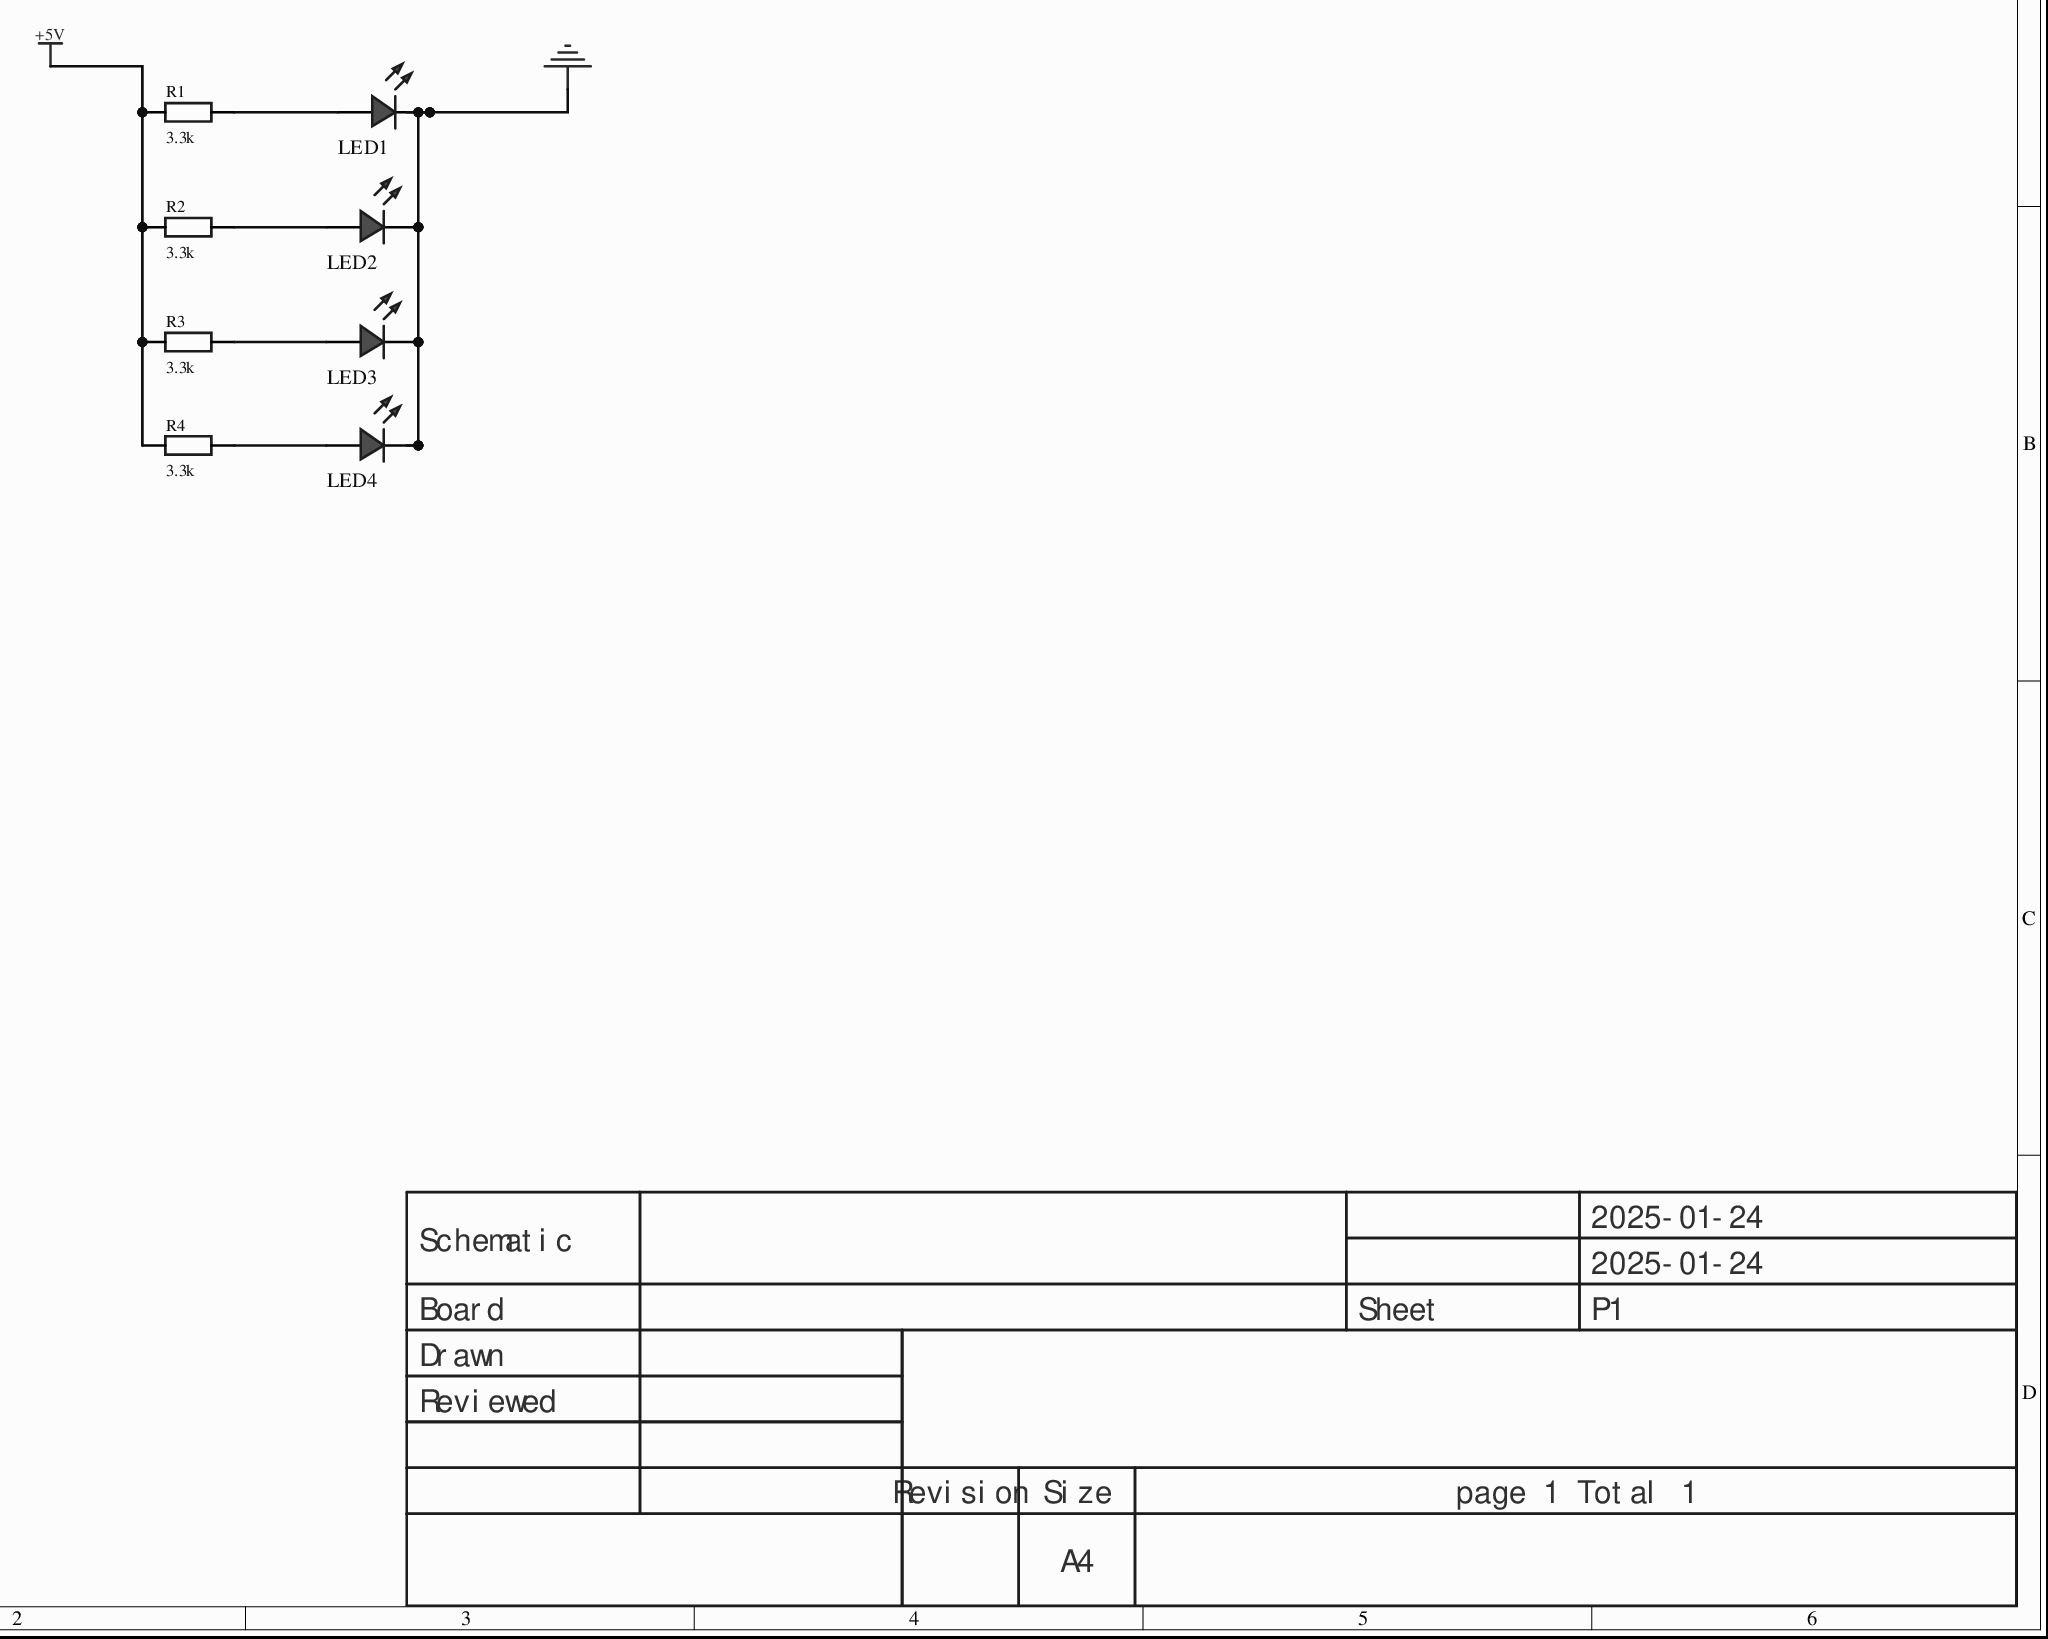
[diagram p0: MISC51832-3.schdoc]
# Altium project MISC51832-2.PrjPcb
1 sheet, 8 parts. Net scope: global (net labels, ports and power ports of the same name join across sheets).
Board file: MISC51832.pcbdoc

## Sheet MISC51832-3.schdoc
size 297 x 209 mm; Version: V1.0; @Project Name: MISC51832; @Page Count: 1; @Update Date: 2025-01-24; @Create Date: 2025-01-24; @Schematic Name: MISC51832; @Page No: 1; @Create Time: 20:13:33; @Update Time: 20:13:33; @Board Name: MISC51832

### Parts
LED1  (no value)  [LED_0603]
LED2  (no value)  [LED_0603]
LED3  (no value)  [LED_0603]
LED4  (no value)  [LED_0603]
R1  3.3k  [R0603]
R2  3.3k  [R0603]
R3  3.3k  [R0603]
R4  3.3k  [R0603]

### Nets
+5V: R1.1 R2.1 R3.1 R4.1
GND: LED1.1(C) LED2.1(C) LED3.1(C) LED4.1(C)
NetLED1_2: LED1.2(A) R1.2
NetLED2_2: LED2.2(A) R2.2
NetLED3_2: LED3.2(A) R3.2
NetLED4_2: LED4.2(A) R4.2

### Notes on the sheet
- 2025-01-24
- Schematic
- Board
- Sheet
- P1
- Drawn
- Reviewed
- Revision
- Size
- A4
- page 1 Total 1

### Library data of the parts
LED1-LED4 = LED_0603-R: Symbol: LED_R; Convert to PCB: yes; 3D Model: dd8257b0d61a4cd7b68939a056e08095; 3D Model Transform: 58.72,29.4,22.03,0,0,0,0,0,0; ModelName: LED-0603_R; Device: LED_0603-R; Add into BOM: yes; Supplier Footprint: 0603; FootprintName: LED_0603
R1-R4 = Res_0603: ConvertToPcb: yes; SymbolName: Resistor; ModelId: fc143cca1e79419f9cd78b61e9279f08; ModelTransform: 31.8897,63.7794,0,90,0,0,0,0,0; Value: 3.3k; Device: Res_0603; AddInBom: yes; Supplier Footprint: 0603; FootprintName: R0603; ModelName: R0603